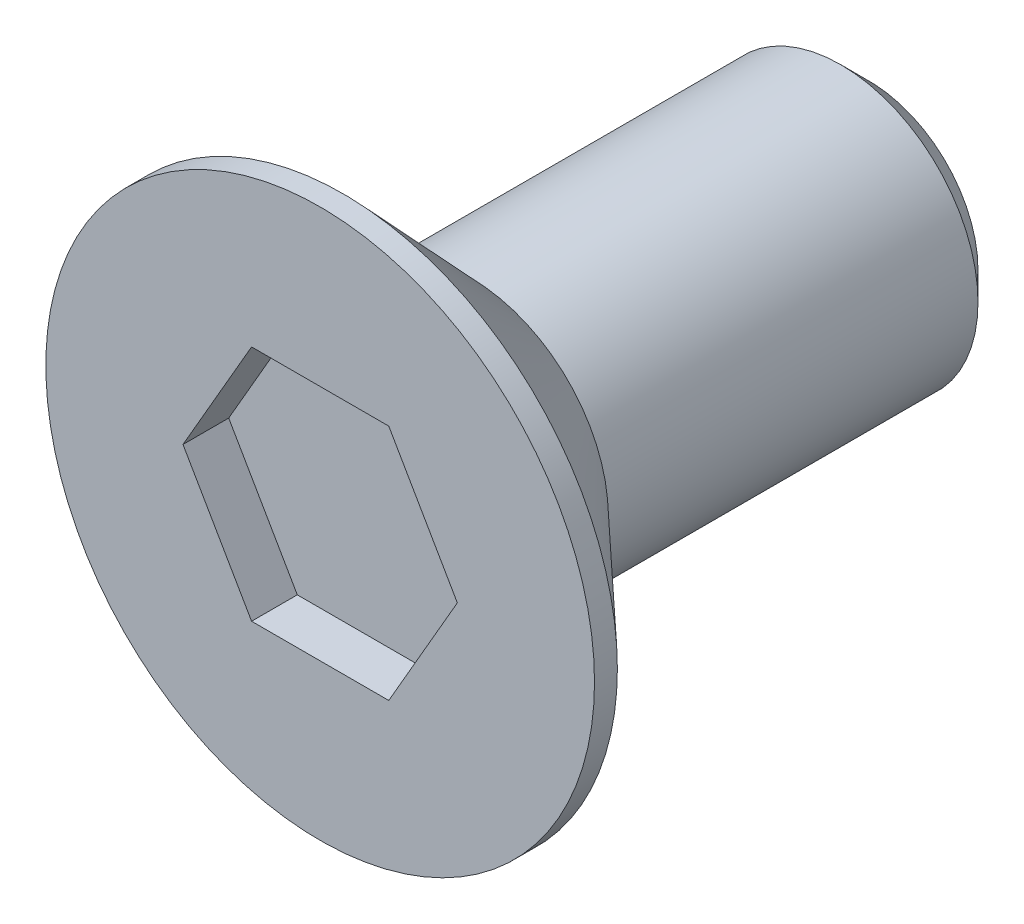
SolidWorks part; units mm, degrees
material "AISI 304"
ref_plane "前视基准面" through (0, 0, 0) normal (0, 0, 1) x (1, 0, 0)
ref_plane "上视基准面" through (0, 0, 0) normal (0, 1, 0) x (1, 0, 0)
ref_plane "右视基准面" through (0, 0, 0) normal (1, 0, 0) x (0, 0, -1)
sketch "草图1" plane through (0, 0, 0) normal (0, 1, 0) x (1, 0, 0)
  line L0 (3, 12) -> (0, 12)
  line L1 (0, 12) -> (0, 0)
  line L2 (0, 0) -> (6, 0)
  line L3 (6, 0) -> (6, 0.5)
  line L4 (6, 0.5) -> (3, 3.3)
  line L5 (3, 3.3) -> (3, 12)
  line L6 (0, 12) -> (0, 0) construction
revolve "旋转1" add sketch "草图1" angle 360 about L6
sketch "草图2" plane through (0, 0, 0) normal (0, 0, 1) x (1, 0, 0)
  line L0 (1.5, -2.5981) -> (3, 0)
  line L1 (3, 0) -> (1.5, 2.5981)
  line L2 (1.5, 2.5981) -> (-1.5, 2.5981)
  line L3 (-1.5, 2.5981) -> (-3, 0)
  line L4 (-3, 0) -> (-1.5, -2.5981)
  line L5 (-1.5, -2.5981) -> (1.5, -2.5981)
extrude "切除-拉伸1" cut sketch "草图2" against normal blind 1
chamfer "倒角1" distance 0.6135 angle 45 1 edges at (3, 0, -12)
